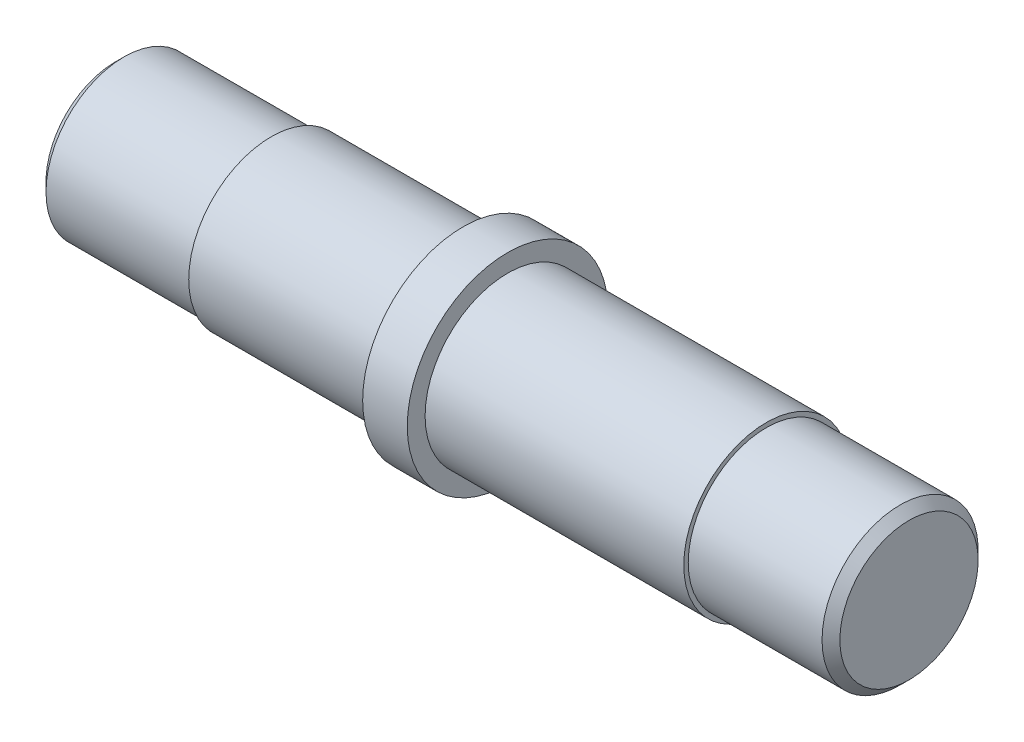
from build123d import *

# Parameters (mm, degrees)
CHAMFER1_SIZE       = 2
CUT_EXTRUDE1_DEPTH  = 88
BOSS_EXTRUDE1_DEPTH = 13.5
SCALE_1_SCALE       = 1.875


with BuildPart() as part:
    # Sketch1 → Revolve1 (revolve)
    with BuildSketch(Plane.XY, mode=Mode.PRIVATE) as revolve1_sk:
        Polygon((-66.093473684, 0), (-66.093473684, 17.5), (-31.093473684, 17.5), (-31.093473684, 18.5), (11.906526316, 18.5), (11.906526316, 22.5), (21.906526316, 22.5), (21.906526316, 18.5), (79.906526316, 18.5), (79.906526316, 17.5), (111.906526316, 17.5), (111.906526316, 0), align=None)
    revolve(revolve1_sk.sketch.rotate(Axis((-66.093473684, 0, 0), (1, 0, 0)), 90), axis=Axis((-66.093473684, 0, 0), (1, 0, 0)))

    # Chamfer1
    chamfer1_edges = [part.edges().sort_by_distance(p)[0] for p in [
        (-66.093473684, 0, -17.5),
        (111.906526316, 0, -17.5),
    ]]
    chamfer(chamfer1_edges, length=CHAMFER1_SIZE)

    # Sketch 2_2 → Cut-Extrude1 (cut)
    with BuildSketch(Plane(origin=(0, 0, 0), x_dir=(1, 0, 0), z_dir=(0, 1, 0))):
        with BuildLine():
            Line((-21.093473684, 4.5), (-0.093473684, 4.5))
            ThreePointArc((-0.093473684, 4.5), (4.406526316, 0), (-0.093473684, -4.5))
            Line((-0.093473684, -4.5), (-21.093473684, -4.5))
            ThreePointArc((-21.093473684, -4.5), (-25.593473684, 0), (-21.093473684, 4.5))
        make_face()
        with BuildLine():
            Line((34.906526316, 4.5), (69.906526316, 4.5))
            ThreePointArc((69.906526316, 4.5), (74.406526316, 0), (69.906526316, -4.5))
            Line((69.906526316, -4.5), (34.906526316, -4.5))
            ThreePointArc((34.906526316, -4.5), (30.406526316, 0), (34.906526316, 4.5))
        make_face()
    extrude(amount=-CUT_EXTRUDE1_DEPTH, mode=Mode.SUBTRACT)

    # Sketch 2_2 2 → Boss-Extrude1 (add)
    with BuildSketch(Plane(origin=(0, 0, 0), x_dir=(1, 0, 0), z_dir=(0, 1, 0))):
        with BuildLine():
            Line((-21.093473684, 4.5), (-0.093473684, 4.5))
            ThreePointArc((-0.093473684, 4.5), (4.406526316, 0), (-0.093473684, -4.5))
            Line((-0.093473684, -4.5), (-21.093473684, -4.5))
            ThreePointArc((-21.093473684, -4.5), (-25.593473684, 0), (-21.093473684, 4.5))
        make_face()
        with BuildLine():
            Line((34.906526316, 4.5), (69.906526316, 4.5))
            ThreePointArc((69.906526316, 4.5), (74.406526316, 0), (69.906526316, -4.5))
            Line((69.906526316, -4.5), (34.906526316, -4.5))
            ThreePointArc((34.906526316, -4.5), (30.406526316, 0), (34.906526316, 4.5))
        make_face()
    extrude(amount=-BOSS_EXTRUDE1_DEPTH)


with BuildPart() as part_1:
    # Scale 1: scaled about (22.77118049, 0.261331354, 1.672e-06)
    add(part.part.scale(SCALE_1_SCALE).moved(Location((-19.924782929, -0.228664935, -1.463e-06))))


solid = part_1.part
